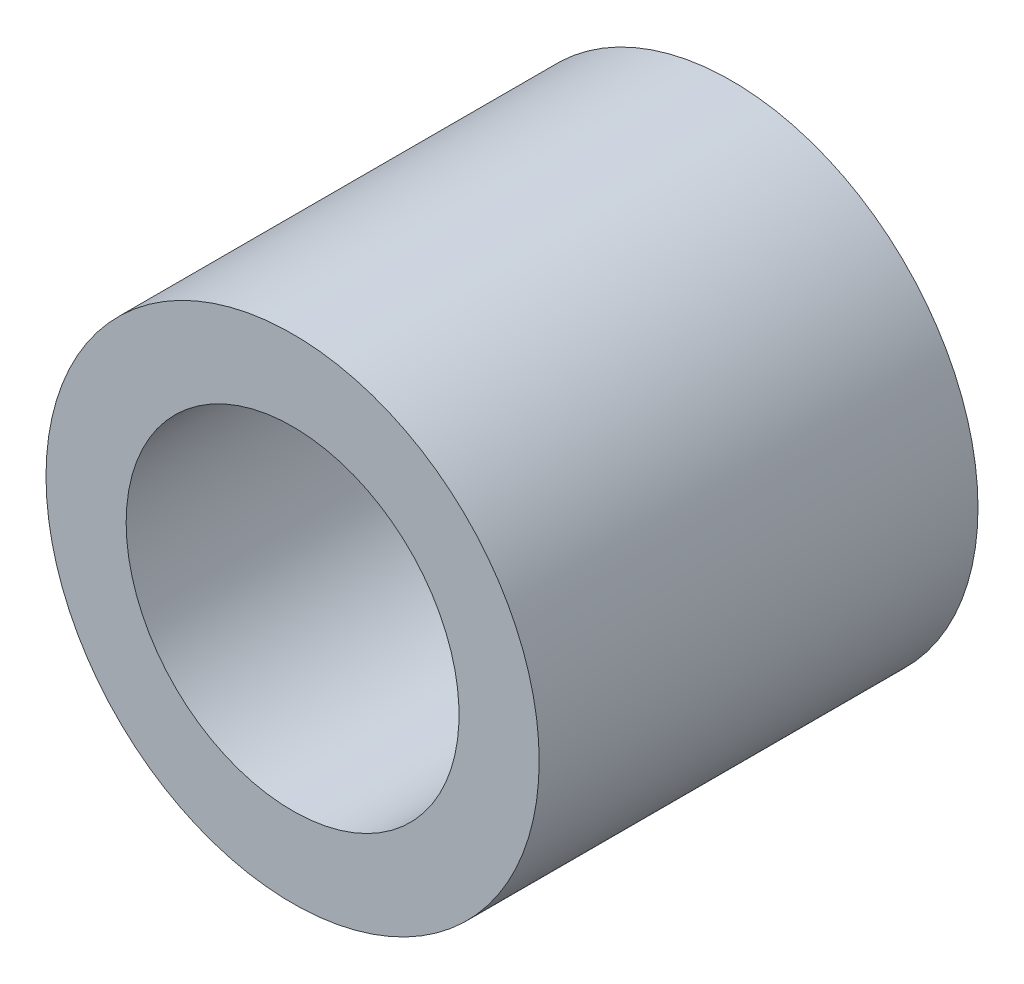
from build123d import *

# Parameters (mm, degrees)
SKETCH1_R           = 6
SKETCH1_R_2         = 4.05
BOSS_EXTRUDE1_DEPTH = 10.676916711


with BuildPart() as part:
    # Sketch1 → Boss-Extrude1 (new body)
    with BuildSketch(Plane.XY):
        with Locations(Location((10, -61.753173354, 0), (0, 0, 180))):
            Circle(SKETCH1_R)
        with Locations(Location((10, -61.753173354, 0), (0, 0, 180))):
            Circle(SKETCH1_R_2, mode=Mode.SUBTRACT)
    extrude(amount=BOSS_EXTRUDE1_DEPTH)


solid = part.part
